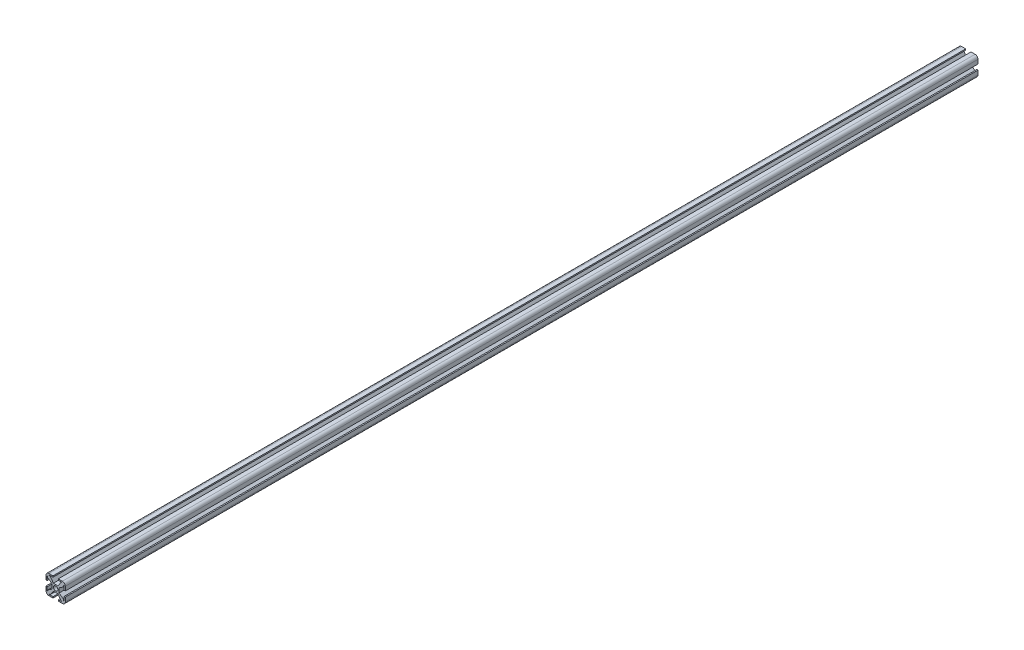
SolidWorks part; units mm, degrees
ref_plane "前视基准面" through (0, 0, 0) normal (0, 0, 1) x (1, 0, 0)
ref_plane "上视基准面" through (0, 0, 0) normal (0, 1, 0) x (1, 0, 0)
ref_plane "右视基准面" through (0, 0, 0) normal (1, 0, 0) x (0, 0, -1)
sketch "草图1" plane through (0, 0, 0) normal (0, 0, 1) x (1, 0, 0)
  line L1 (15, -15) -> (-15, -15)
  line L2 (15, -15) -> (15, 15)
  line L3 (15, 15) -> (-15, 15)
  line L4 (-15, -15) -> (-15, 15)
  line L5 (15, -15) -> (-15, 15) construction
  line L6 (15, 15) -> (-15, -15) construction
  point P0 (0, 0)
  dimension "D1" = 30
extrude "凸台-拉伸1" add sketch "草图1" along normal mid plane 1420
fillet "圆角1" radius 4.5 4 edges at (15, -15, 0) (15, 15, 0) (-15, 15, 0) (-15, -15, 0)
sketch "草图2" plane through (0, 0, 710) normal (0, 0, 1) x (1, 0, 0)
  line L0 (10.5, 15) -> (-10.5, 15) construction
  line L1 (4.1, 17.2) -> (-4.1, 17.2)
  line L2 (4.1, 17.2) -> (4.1, 12.8)
  line L3 (4.1, 12.8) -> (-4.1, 12.8)
  line L4 (-4.1, 17.2) -> (-4.1, 12.8)
  line L5 (4.1, 17.2) -> (-4.1, 12.8) construction
  line L6 (4.1, 12.8) -> (-4.1, 17.2) construction
  line L7 (-10.25, 12.5) -> (-5.3, 5.3)
  line L8 (10.25, 13.1) -> (-10.25, 13.1)
  line L9 (10.25, 13.1) -> (10.25, 12.5)
  line L10 (10.25, 12.5) -> (-10.25, 12.5)
  line L11 (-10.25, 13.1) -> (-10.25, 12.5)
  line L12 (10.25, 13.1) -> (-10.25, 12.5) construction
  line L13 (10.25, 12.5) -> (-10.25, 13.1) construction
  line L14 (5.3, -5.3) -> (-5.3, -5.3)
  line L15 (5.3, -5.3) -> (5.3, 5.3)
  line L16 (5.3, 5.3) -> (-5.3, 5.3)
  line L17 (-5.3, -5.3) -> (-5.3, 5.3)
  line L18 (5.3, -5.3) -> (-5.3, 5.3) construction
  line L19 (5.3, 5.3) -> (-5.3, -5.3) construction
  line L20 (-8.4297, 12.5) -> (-3.4797, 5.3)
  line L21 (10.25, 12.5) -> (5.3, 5.3)
  line L22 (8.4297, 12.5) -> (3.4797, 5.3)
  circle A0 centre (0, 0) radius 3.4
  point P0 (0, 15)
  point P7 (0, 12.8)
  point P12 (0, 0)
  line M7 (10.5, 15) -> (-10.5, 15)
  dimension "D6" = 6.8
  dimension "D1" = 8.2
  dimension "D2" = 20.5
  dimension "D3" = 10.6
  dimension "D4" = 1.5
  dimension "D5" = 1.5
  dimension "D7" = 1.9
  dimension "D8" = 12.5
extrude "切除-拉伸1" cut sketch "草图2" against normal through all contours L2 L8 L4 L3 | L8 L2 L4 M7 | L8 L11 L10 L9 L2 L3 L4 | L22 L10 L20 L16 | A0
pattern_circular "阵列(圆周)1" count 4 over 360 about axis through (0, 0, 0) along (0, 0, 1) of "切除-拉伸1"
